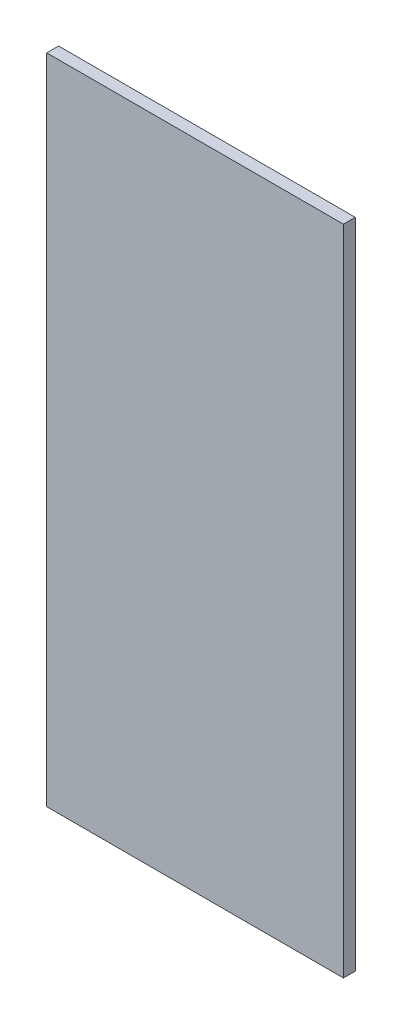
from build123d import *

# Parameters (mm, degrees)
SKETCH_1_W      = 50
SKETCH_1_H      = 110
EXTRUDE_1_DEPTH = 1


with BuildPart() as part:
    # 草图1 → 凸台-拉伸1 (new, symmetric)
    with BuildSketch(Plane.XY):
        Rectangle(SKETCH_1_W, SKETCH_1_H)
    extrude(amount=EXTRUDE_1_DEPTH, both=True)


solid = part.part
